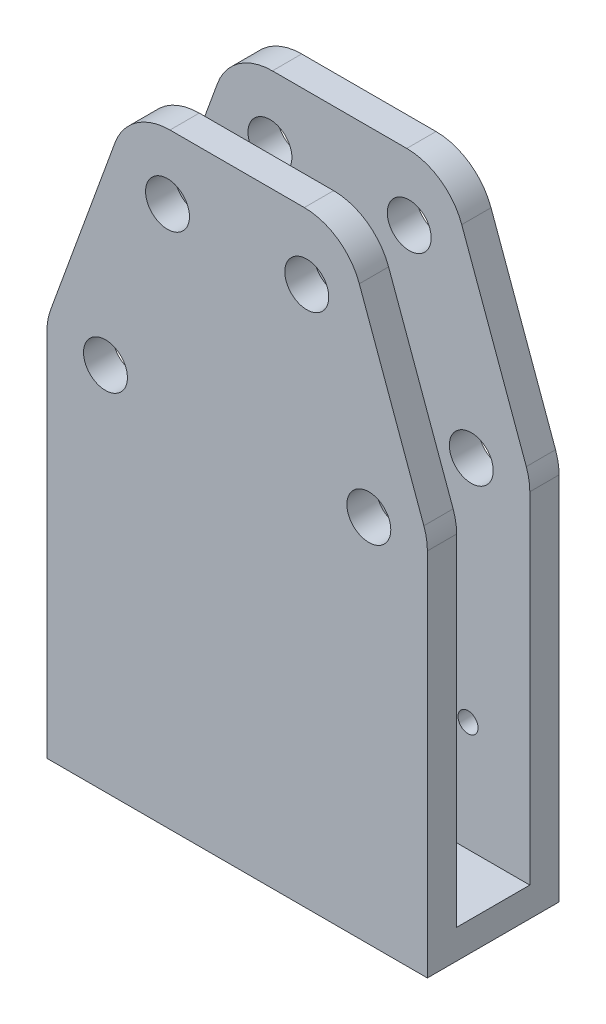
from build123d import *

# Parameters (mm, degrees)
BOSS_EXTRUDE1_DEPTH            = 10
SKETCH2_W                      = 130
SKETCH2_H                      = 10
BOSS_EXTRUDE2_DEPTH            = 25
BOSS_EXTRUDE3_DEPTH            = 10
CUT_EXTRUDE1_DEPTH             = 5
CUT_EXTRUDE2_START             = -5
CUT_EXTRUDE2_DEPTH             = 5
F_15_0_15_DIAMETER_HOLE1_D     = 15
F_15_0_15_DIAMETER_HOLE1_DEPTH = 10
HOLE1_D                        = 5.1881
HOLE1_DEPTH                    = 10
F_15_0_15_DIAMETER_HOLE2_D     = 15
F_15_0_15_DIAMETER_HOLE2_DEPTH = 45
FILLET1_R                      = 5
FILLET2_R                      = 20
SCALE1_SCALE                   = 0.3
SKETCH14_W                     = 19.347729644
SKETCH14_H                     = 16.426581325
BOSS_EXTRUDE4_DEPTH            = 3
M2_5_TAPPED_HOLE1_D            = 2.05
M2_5_TAPPED_HOLE1_DEPTH        = 6.35
M2_5_TAPPED_HOLE1_TIP          = 0.615882135
M5_TAPPED_HOLE1_D              = 4.2


with BuildPart() as part:
    # Sketch1 → Boss-Extrude1 (new body)
    with BuildSketch(Plane.XY.offset(10)):
        Polygon((-65, 200), (-65, 70.093194396), (65, 70.093194396), (65, 200), (36.954348247, 277.054794904), (-36.954348247, 277.054794904), align=None)
    extrude(amount=-BOSS_EXTRUDE1_DEPTH)

    # Sketch2 → Boss-Extrude2 (add)
    with BuildSketch(Plane.XY.offset(10)):
        with Locations((0, 75.093194396)):
            Rectangle(SKETCH2_W, SKETCH2_H)
    extrude(amount=BOSS_EXTRUDE2_DEPTH)

    # Sketch3 → Boss-Extrude3 (add)
    with BuildSketch(Plane.XY.offset(35)):
        Polygon((-65, 70.093194396), (-65, 200), (-36.954348247, 277.054794904), (36.954348247, 277.054794904), (65, 200), (65, 70.093194396), align=None)
    extrude(amount=BOSS_EXTRUDE3_DEPTH)

    # Sketch4 → Cut-Extrude1 (cut)
    with BuildSketch(Plane(origin=(0, 0, 35), x_dir=(-1, 0, 0), z_dir=(0, 0, -1))):
        with BuildLine():
            Line((-18.045302576, 207.054794904), (18.045302576, 207.054794904))
            ThreePointArc((18.045302576, 207.054794904), (22.141062797, 209.186912723), (22.743765679, 213.764895621))
            Line((22.743765679, 213.764895621), (12.44708441, 242.054794904))
            Line((12.44708441, 242.054794904), (-12.44708441, 242.054794904))
            Line((-12.44708441, 242.054794904), (-22.743765679, 213.764895621))
            ThreePointArc((-22.743765679, 213.764895621), (-22.141062797, 209.186912723), (-18.045302576, 207.054794904))
        make_face()
    extrude(amount=-CUT_EXTRUDE1_DEPTH, mode=Mode.SUBTRACT)

    # Sketch5 → Cut-Extrude2 (cut)
    with BuildSketch(Plane.XY.offset(10).offset(CUT_EXTRUDE2_START)):
        with BuildLine():
            Line((22.743765679, 213.764895621), (12.44708441, 242.054794904))
            Line((12.44708441, 242.054794904), (-12.44708441, 242.054794904))
            Line((-12.44708441, 242.054794904), (-22.743765679, 213.764895621))
            ThreePointArc((-22.743765679, 213.764895621), (-22.141062797, 209.186912723), (-18.045302576, 207.054794904))
            Line((-18.045302576, 207.054794904), (18.045302576, 207.054794904))
            ThreePointArc((18.045302576, 207.054794904), (22.141062797, 209.186912723), (22.743765679, 213.764895621))
        make_face()
    extrude(amount=CUT_EXTRUDE2_DEPTH, mode=Mode.SUBTRACT)

    # Ø15.0 (15) Diameter Hole1
    with Locations(Plane.XY.offset(45)):
        with Locations((8.888888889, 130.739240574), (45, 196.473460386), (-45, 196.473460386), (-23.794751114, 254.734402875), (23.794751114, 254.734402875)):
            Hole(F_15_0_15_DIAMETER_HOLE1_D / 2, depth=F_15_0_15_DIAMETER_HOLE1_DEPTH)

    # Hole1
    with Locations(Plane.XY.offset(45)):
        with Locations((-9.311866244, 122.448733195), (0.59838151, 148.939995706), (27.089644022, 139.029747952), (17.179396267, 112.538485441)):
            Hole(HOLE1_D / 2, depth=HOLE1_DEPTH)

    # Ø15.0 (15) Diameter Hole2
    with Locations(Plane(origin=(0, 0, 0), x_dir=(-1, 0, 0), z_dir=(0, 0, -1))):
        with Locations((-8.888888889, 130.739240574), (-45, 196.473460386), (45, 196.473460386), (23.794751114, 254.734402875), (-23.794751114, 254.734402875)):
            Hole(F_15_0_15_DIAMETER_HOLE2_D / 2, depth=F_15_0_15_DIAMETER_HOLE2_DEPTH)

    # Fillet1
    fillet1_edges = [part.edges().sort_by_distance(p)[0] for p in [
        (12.44708441, 242.054794904, 37.5),
        (-12.44708441, 242.054794904, 37.5),
        (-12.44708441, 242.054794904, 7.5),
        (12.44708441, 242.054794904, 7.5),
    ]]
    fillet(fillet1_edges, radius=FILLET1_R)

    # Fillet2
    fillet2_edges = [part.edges().sort_by_distance(p)[0] for p in [
        (-36.954348247, 277.054794904, 5),
        (36.954348247, 277.054794904, 5),
        (65, 200, 5),
        (-65, 200, 5),
        (65, 200, 40),
        (36.954348247, 277.054794904, 40),
        (-36.954348247, 277.054794904, 40),
        (-65, 200, 40),
    ]]
    fillet(fillet2_edges, radius=FILLET2_R)


with BuildPart() as part_1:
    # Scale1: scaled about (0, 0, 0)
    add(part.part.scale(SCALE1_SCALE))

    # Sketch14 → Boss-Extrude4 (add)
    with BuildSketch(Plane.XY.offset(13.5)):
        with Locations((2.169151432, 38.275577148)):
            Rectangle(SKETCH14_W, SKETCH14_H)
    extrude(amount=-BOSS_EXTRUDE4_DEPTH)

    # M2.5 Tapped Hole1
    with Locations(Plane(origin=(0, 0, 0), x_dir=(-1, 0, 0), z_dir=(0, 0, -1))):
        with Locations((7.833333333, 35.321772172), (-13.166666667, 35.321772172)):
            Hole(M2_5_TAPPED_HOLE1_D / 2, depth=M2_5_TAPPED_HOLE1_DEPTH)
            with Locations((0, 0, -(M2_5_TAPPED_HOLE1_DEPTH + M2_5_TAPPED_HOLE1_TIP / 2))):  # 118° drill point
                Cone(0, M2_5_TAPPED_HOLE1_D / 2, M2_5_TAPPED_HOLE1_TIP, mode=Mode.SUBTRACT)

    # M5 Tapped Hole1 (through all)
    with Locations(Plane(origin=(0, 21.027958319, 0), x_dir=(-1, 0, 0), z_dir=(0, -1, 0))):
        with Locations((12.5, -6.75), (-12.5, -6.75)):
            Hole(M5_TAPPED_HOLE1_D / 2)


solid = part_1.part
